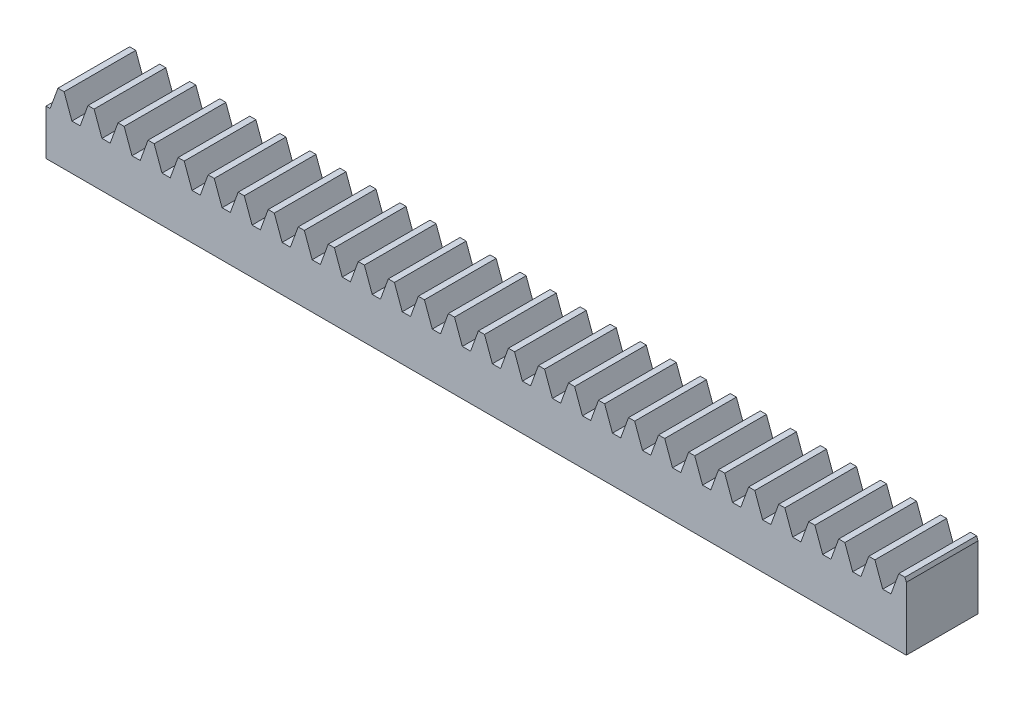
from build123d import *

# Parameters (mm, degrees)
BLANKSKE_W        = 180
BLANKSKE_H        = 14
BLANK_DEPTH       = 15
TOOTHCUTSIM_DEPTH = 182.165670037
TEETHCUTS_COUNT   = 30
TEETHCUTS_PITCH   = 6.2831853


with BuildPart() as part:
    # BlankSke → Blank (new body)
    with BuildSketch(Plane.XY):
        with Locations((90, 7)):
            Rectangle(BLANKSKE_W, BLANKSKE_H)
    extrude(amount=-BLANK_DEPTH)

    # TooCutSkeSim → ToothCutSim (cut, through all)
    with BuildSketch(Plane.XY):
        Polygon((0.861870739, 9.5), (-0.861870739, 9.5), (-2.508981637, 14.0254), (2.508981637, 14.0254), align=None)
    toothcutsim = extrude(amount=-TOOTHCUTSIM_DEPTH, mode=Mode.SUBTRACT)

    # TeethCuts: ToothCutSim ×30
    with Locations(*[(i * TEETHCUTS_PITCH, 0, 0) for i in range(1, TEETHCUTS_COUNT)]):
        add(toothcutsim, mode=Mode.SUBTRACT)


solid = part.part
